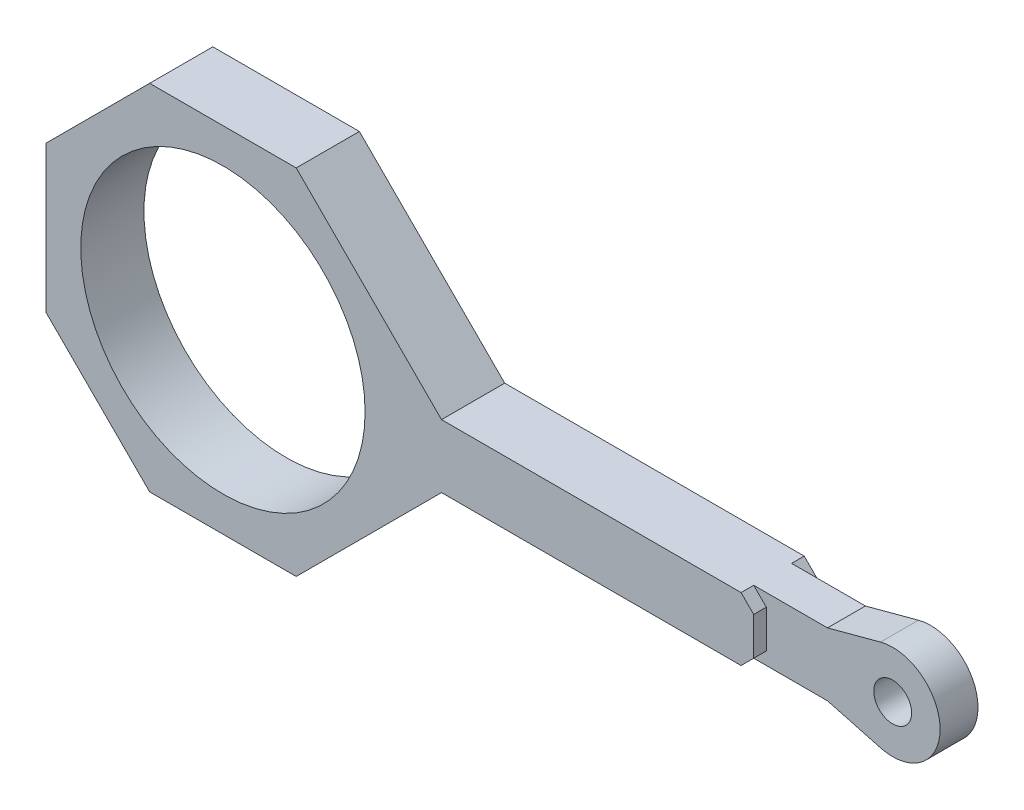
from build123d import *

# Parameters (mm, degrees)
SKETCH_1_3_R        = 22.5
BOSS_EXTRUDE1_DEPTH = 5
BOSS_EXTRUDE2_DEPTH = 3
SKETCH2_R           = 3
CUT_EXTRUDE1_DEPTH  = 15.5


with BuildPart() as part:
    # Sketch 1_3 → Boss-Extrude1 (new, symmetric)
    with BuildSketch(Plane.XY):
        Polygon((34.597979746, 5), (28, 11.597979746), (11.597979746, 28), (-11.597979746, 28), (-28, 11.597979746), (-28, -11.597979746), (-11.597979746, -28), (11.597979746, -28), (19.798989873, -19.798989873), (28, -11.597979746), (34.597979746, -5), (82, -5), (84, -3), (84, 3), (82, 5), align=None)
        Circle(SKETCH_1_3_R, mode=Mode.SUBTRACT)
    extrude(amount=BOSS_EXTRUDE1_DEPTH, both=True)

    # Sketch 1_3 2 → Boss-Extrude2 (add, symmetric)
    with BuildSketch(Plane.XY):
        with BuildLine():
            Line((93.682479249, 5), (82, 5))
            Line((82, 5), (84, 3))
            Line((84, 3), (84, -3))
            Line((84, -3), (82, -5))
            Line((82, -5), (93.682479249, -5))
            Line((93.682479249, -5), (102.058857162, -7.244443697))
            ThreePointArc((102.058857162, -7.244443697), (111.5, 0), (102.058857162, 7.244443697))
            Line((102.058857162, 7.244443697), (93.682479249, 5))
        make_face()
    extrude(amount=BOSS_EXTRUDE2_DEPTH, both=True)

    # Sketch2 → Cut-Extrude1 (cut, symmetric)
    with BuildSketch(Plane.XY.offset(3)):
        with Locations((104, 0)):
            Circle(SKETCH2_R)
    extrude(amount=CUT_EXTRUDE1_DEPTH, both=True, mode=Mode.SUBTRACT)


solid = part.part
